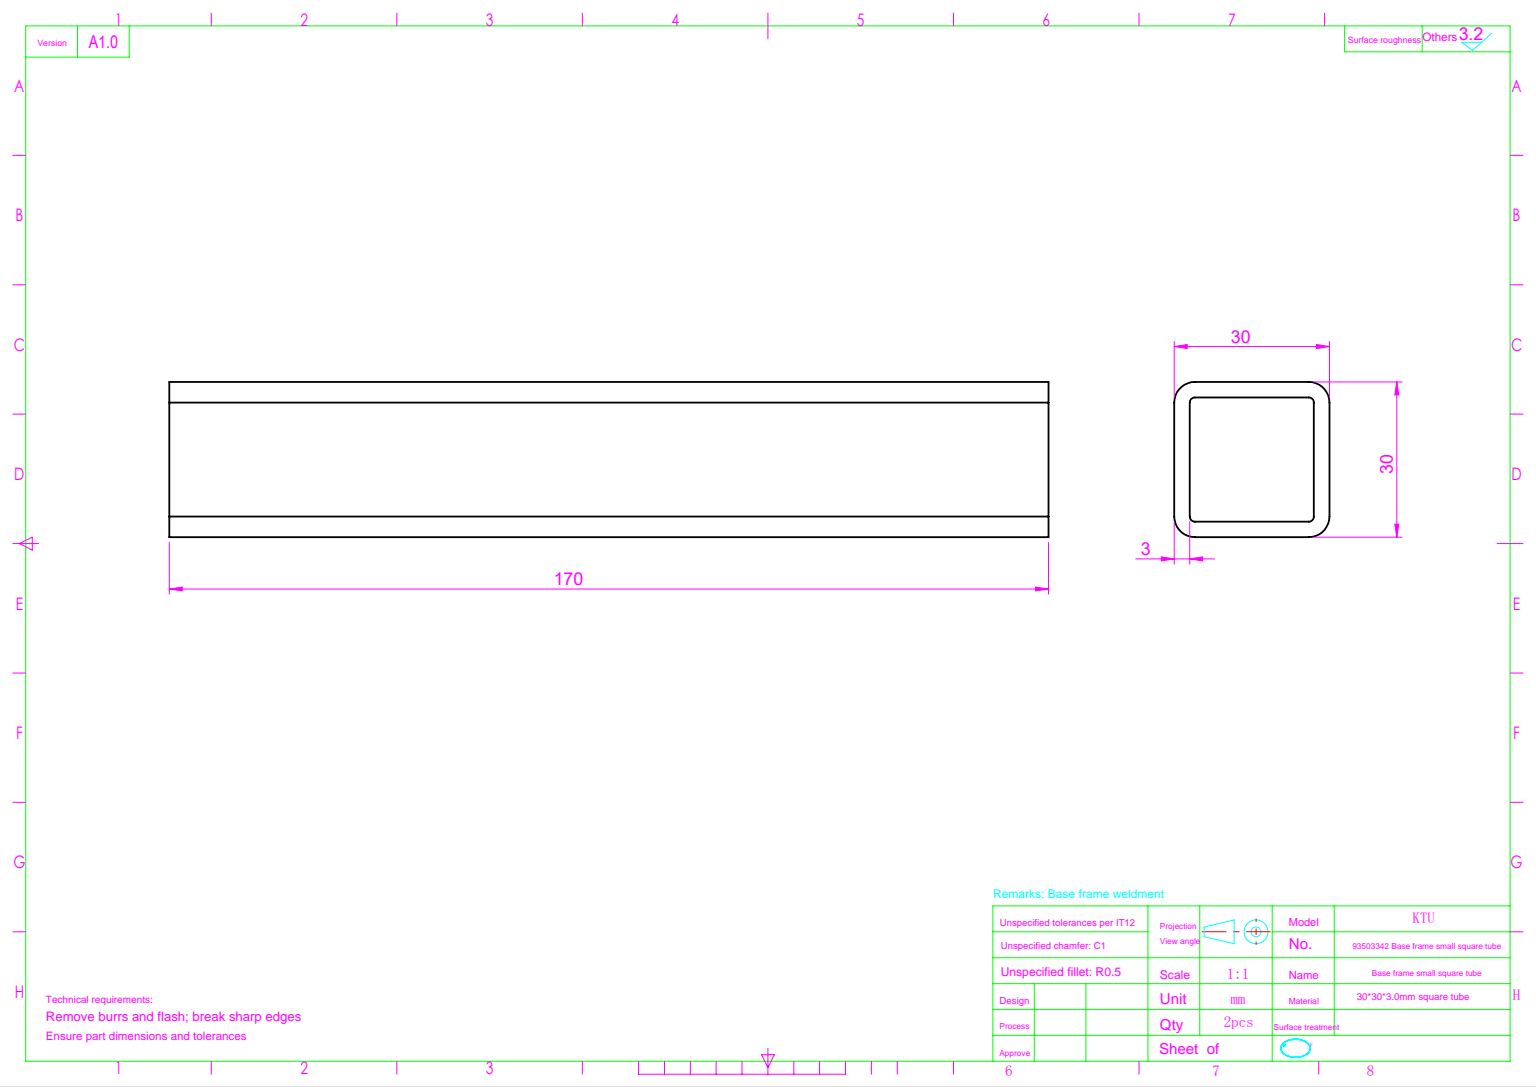
from build123d import *

# Parameters (mm, degrees)
EXTRUDE_1_DEPTH = 85


with BuildPart() as part:
    # 草图2 → 拉伸-薄壁1 (new, symmetric)
    with BuildSketch(Plane.XY):
        with BuildLine():
            Line((-11, 15), (11, 15))
            ThreePointArc((11, 15), (13.828427125, 13.828427125), (15, 11))
            Line((15, 11), (15, -11))
            ThreePointArc((15, -11), (13.828427125, -13.828427125), (11, -15))
            Line((11, -15), (-11, -15))
            ThreePointArc((-11, -15), (-13.828427125, -13.828427125), (-15, -11))
            Line((-15, -11), (-15, 11))
            ThreePointArc((-15, 11), (-13.828427125, 13.828427125), (-11, 15))
        make_face()
        with BuildLine():
            Line((-11, 12), (11, 12))
            ThreePointArc((11, 12), (11.707106781, 11.707106781), (12, 11))
            Line((12, 11), (12, -11))
            ThreePointArc((12, -11), (11.707106781, -11.707106781), (11, -12))
            Line((11, -12), (-11, -12))
            ThreePointArc((-11, -12), (-11.707106781, -11.707106781), (-12, -11))
            Line((-12, -11), (-12, 11))
            ThreePointArc((-12, 11), (-11.707106781, 11.707106781), (-11, 12))
        make_face(mode=Mode.SUBTRACT)
    extrude(amount=EXTRUDE_1_DEPTH, both=True)


solid = part.part
